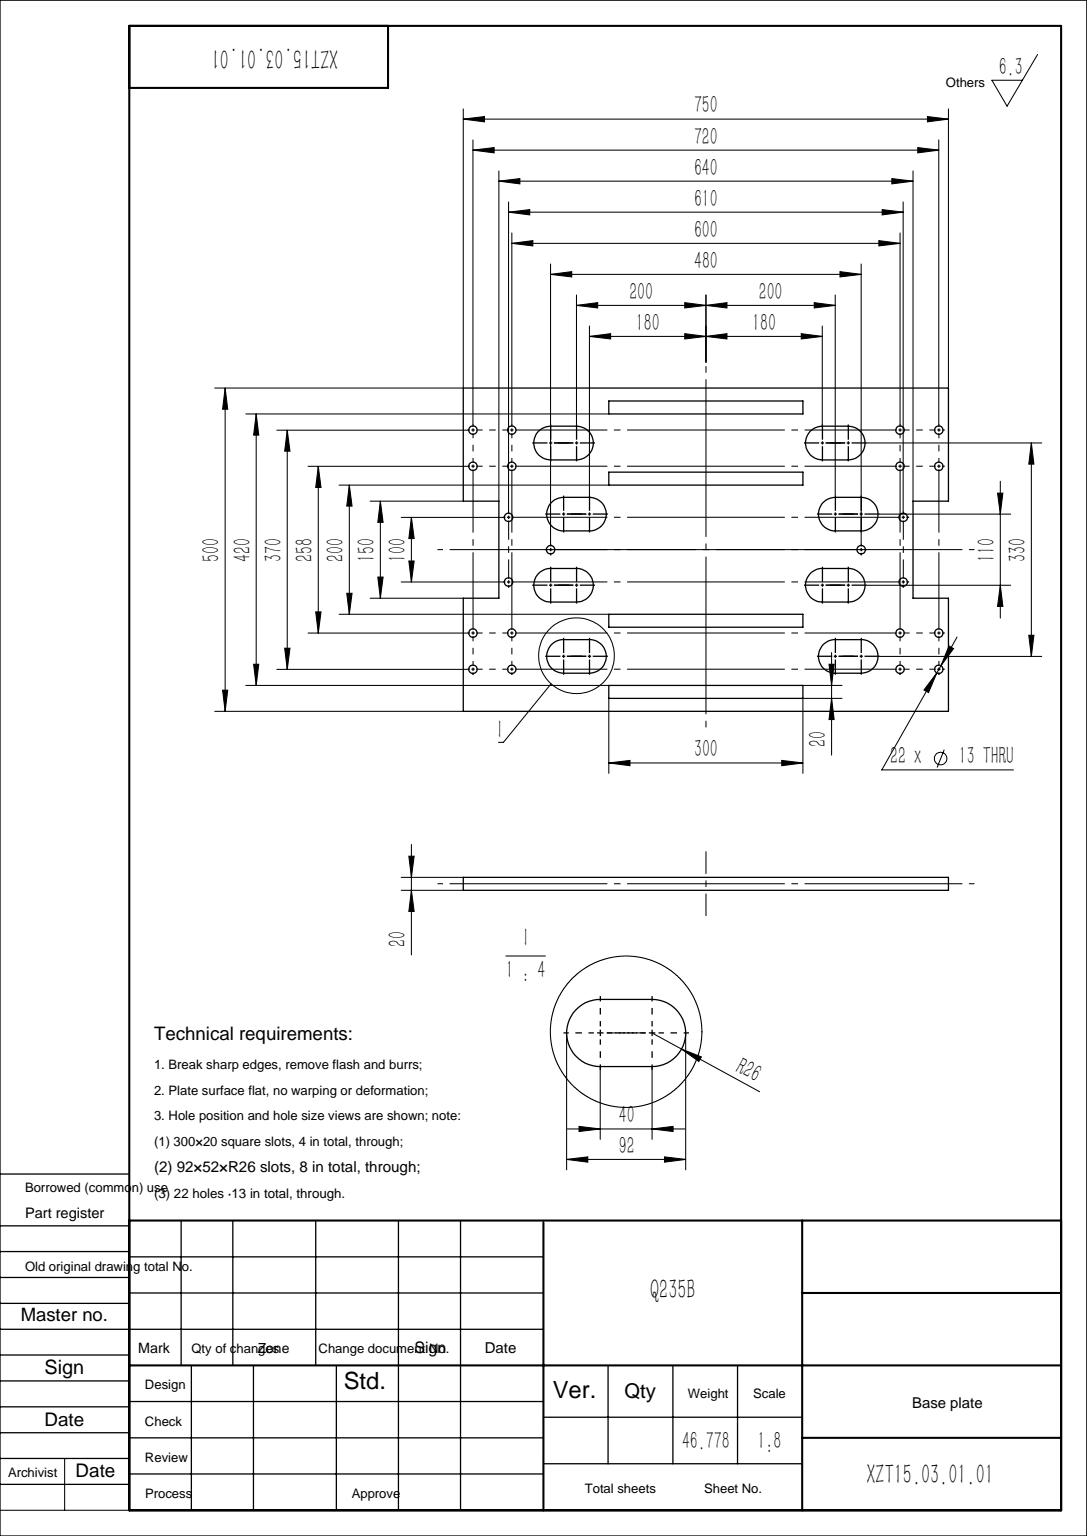
from build123d import *

# Parameters (mm, degrees)
SKETCH1_W                  = 300
SKETCH1_H                  = 20
BOSS_EXTRUDE1_DEPTH        = 20
F_13_0_13_DIAMETER_HOLE1_D = 13
CUT_EXTRUDE1_REACH         = 453.137


with BuildPart() as part:
    # Sketch1 → Boss-Extrude1 (new body)
    with BuildSketch(Plane(origin=(0, 0, 0), x_dir=(1, 0, 0), z_dir=(0, 1, 0))):
        Polygon((-375, -250), (375, -250), (375, -75), (320, -75), (320, 75), (375, 75), (375, 250), (-375, 250), (-375, 75), (-320, 75), (-320, -75), (-375, -75), align=None)
        with Locations((0, -220)):
            Rectangle(SKETCH1_W, SKETCH1_H, mode=Mode.SUBTRACT)
        with Locations((0, -110)):
            Rectangle(SKETCH1_W, SKETCH1_H, mode=Mode.SUBTRACT)
        with Locations((0, 110)):
            Rectangle(SKETCH1_W, SKETCH1_H, mode=Mode.SUBTRACT)
        with Locations((0, 220)):
            Rectangle(SKETCH1_W, SKETCH1_H, mode=Mode.SUBTRACT)
    extrude(amount=BOSS_EXTRUDE1_DEPTH)

    # Ø13.0 (13) Diameter Hole1 (through all)
    with Locations(Plane(origin=(0, 20, 0), x_dir=(1, 0, 0), z_dir=(0, 1, 0))):
        with Locations((-360, 129), (-305, 50), (-240, 0), (-300, 129), (-300, 185), (-360, 185), (-360, -129), (-360, -185), (-300, -129), (-300, -185), (-305, -50), (360, -129), (300, -129), (360, -185), (360, 129), (360, 185), (300, 129), (305, -50), (300, -185), (300, 185), (240, 0), (305, 50)):
            Hole(F_13_0_13_DIAMETER_HOLE1_D / 2)

    # Sketch4 → Cut-Extrude1 (cut, up to next)
    with BuildSketch(Plane(origin=(0, 20, 0), x_dir=(1, 0, 0), z_dir=(0, 1, 0)), mode=Mode.PRIVATE) as cut_extrude1_sk1:
        with BuildLine():
            Line((-240, 191), (-200, 191))
            ThreePointArc((-200, 191), (-174, 165), (-200, 139))
            Line((-200, 139), (-240, 139))
            ThreePointArc((-240, 139), (-266, 165), (-240, 191))
        make_face()
    cut_extrude1_tool1 = extrude(cut_extrude1_sk1.sketch, amount=-CUT_EXTRUDE1_REACH, mode=Mode.PRIVATE) & part.part
    # Sketch4 → Cut-Extrude1 (cut, up to next)
    with BuildSketch(Plane(origin=(0, 20, 0), x_dir=(1, 0, 0), z_dir=(0, 1, 0)), mode=Mode.PRIVATE) as cut_extrude1_sk2:
        with BuildLine():
            Line((-220, 81), (-180, 81))
            ThreePointArc((-180, 81), (-154, 55), (-180, 29))
            Line((-180, 29), (-220, 29))
            ThreePointArc((-220, 29), (-246, 55), (-220, 81))
        make_face()
    cut_extrude1_tool2 = extrude(cut_extrude1_sk2.sketch, amount=-CUT_EXTRUDE1_REACH, mode=Mode.PRIVATE) & part.part
    # Sketch4 → Cut-Extrude1 (cut, up to next)
    with BuildSketch(Plane(origin=(0, 20, 0), x_dir=(1, 0, 0), z_dir=(0, 1, 0)), mode=Mode.PRIVATE) as cut_extrude1_sk3:
        with BuildLine():
            Line((180, 191), (220, 191))
            ThreePointArc((220, 191), (246, 165), (220, 139))
            Line((220, 139), (180, 139))
            ThreePointArc((180, 139), (154, 165), (180, 191))
        make_face()
    cut_extrude1_tool3 = extrude(cut_extrude1_sk3.sketch, amount=-CUT_EXTRUDE1_REACH, mode=Mode.PRIVATE) & part.part
    # Sketch4 → Cut-Extrude1 (cut, up to next)
    with BuildSketch(Plane(origin=(0, 20, 0), x_dir=(1, 0, 0), z_dir=(0, 1, 0)), mode=Mode.PRIVATE) as cut_extrude1_sk4:
        with BuildLine():
            Line((200, 81), (240, 81))
            ThreePointArc((240, 81), (266, 55), (240, 29))
            Line((240, 29), (200, 29))
            ThreePointArc((200, 29), (174, 55), (200, 81))
        make_face()
    cut_extrude1_tool4 = extrude(cut_extrude1_sk4.sketch, amount=-CUT_EXTRUDE1_REACH, mode=Mode.PRIVATE) & part.part
    # Sketch4 → Cut-Extrude1 (cut, up to next)
    with BuildSketch(Plane(origin=(0, 20, 0), x_dir=(1, 0, 0), z_dir=(0, 1, 0)), mode=Mode.PRIVATE) as cut_extrude1_sk5:
        with BuildLine():
            Line((180, -29), (220, -29))
            ThreePointArc((220, -29), (246, -55), (220, -81))
            Line((220, -81), (180, -81))
            ThreePointArc((180, -81), (154, -55), (180, -29))
        make_face()
    cut_extrude1_tool5 = extrude(cut_extrude1_sk5.sketch, amount=-CUT_EXTRUDE1_REACH, mode=Mode.PRIVATE) & part.part
    # Sketch4 → Cut-Extrude1 (cut, up to next)
    with BuildSketch(Plane(origin=(0, 20, 0), x_dir=(1, 0, 0), z_dir=(0, 1, 0)), mode=Mode.PRIVATE) as cut_extrude1_sk6:
        with BuildLine():
            Line((200, -139), (240, -139))
            ThreePointArc((240, -139), (266, -165), (240, -191))
            Line((240, -191), (200, -191))
            ThreePointArc((200, -191), (174, -165), (200, -139))
        make_face()
    cut_extrude1_tool6 = extrude(cut_extrude1_sk6.sketch, amount=-CUT_EXTRUDE1_REACH, mode=Mode.PRIVATE) & part.part
    # Sketch4 → Cut-Extrude1 (cut, up to next)
    with BuildSketch(Plane(origin=(0, 20, 0), x_dir=(1, 0, 0), z_dir=(0, 1, 0)), mode=Mode.PRIVATE) as cut_extrude1_sk7:
        with BuildLine():
            Line((-240, -29), (-200, -29))
            ThreePointArc((-200, -29), (-174, -55), (-200, -81))
            Line((-200, -81), (-240, -81))
            ThreePointArc((-240, -81), (-266, -55), (-240, -29))
        make_face()
    cut_extrude1_tool7 = extrude(cut_extrude1_sk7.sketch, amount=-CUT_EXTRUDE1_REACH, mode=Mode.PRIVATE) & part.part
    # Sketch4 → Cut-Extrude1 (cut, up to next)
    with BuildSketch(Plane(origin=(0, 20, 0), x_dir=(1, 0, 0), z_dir=(0, 1, 0)), mode=Mode.PRIVATE) as cut_extrude1_sk8:
        with BuildLine():
            Line((-220, -139), (-180, -139))
            ThreePointArc((-180, -139), (-154, -165), (-180, -191))
            Line((-180, -191), (-220, -191))
            ThreePointArc((-220, -191), (-246, -165), (-220, -139))
        make_face()
    cut_extrude1_tool8 = extrude(cut_extrude1_sk8.sketch, amount=-CUT_EXTRUDE1_REACH, mode=Mode.PRIVATE) & part.part
    add(cut_extrude1_tool1.solids().sort_by_distance((-220, 20, -165))[0], mode=Mode.SUBTRACT)
    add(cut_extrude1_tool2.solids().sort_by_distance((-200, 20, -55))[0], mode=Mode.SUBTRACT)
    add(cut_extrude1_tool3.solids().sort_by_distance((200, 20, -165))[0], mode=Mode.SUBTRACT)
    add(cut_extrude1_tool4.solids().sort_by_distance((220, 20, -55))[0], mode=Mode.SUBTRACT)
    add(cut_extrude1_tool5.solids().sort_by_distance((200, 20, 55))[0], mode=Mode.SUBTRACT)
    add(cut_extrude1_tool6.solids().sort_by_distance((220, 20, 165))[0], mode=Mode.SUBTRACT)
    add(cut_extrude1_tool7.solids().sort_by_distance((-220, 20, 55))[0], mode=Mode.SUBTRACT)
    add(cut_extrude1_tool8.solids().sort_by_distance((-200, 20, 165))[0], mode=Mode.SUBTRACT)


solid = part.part
